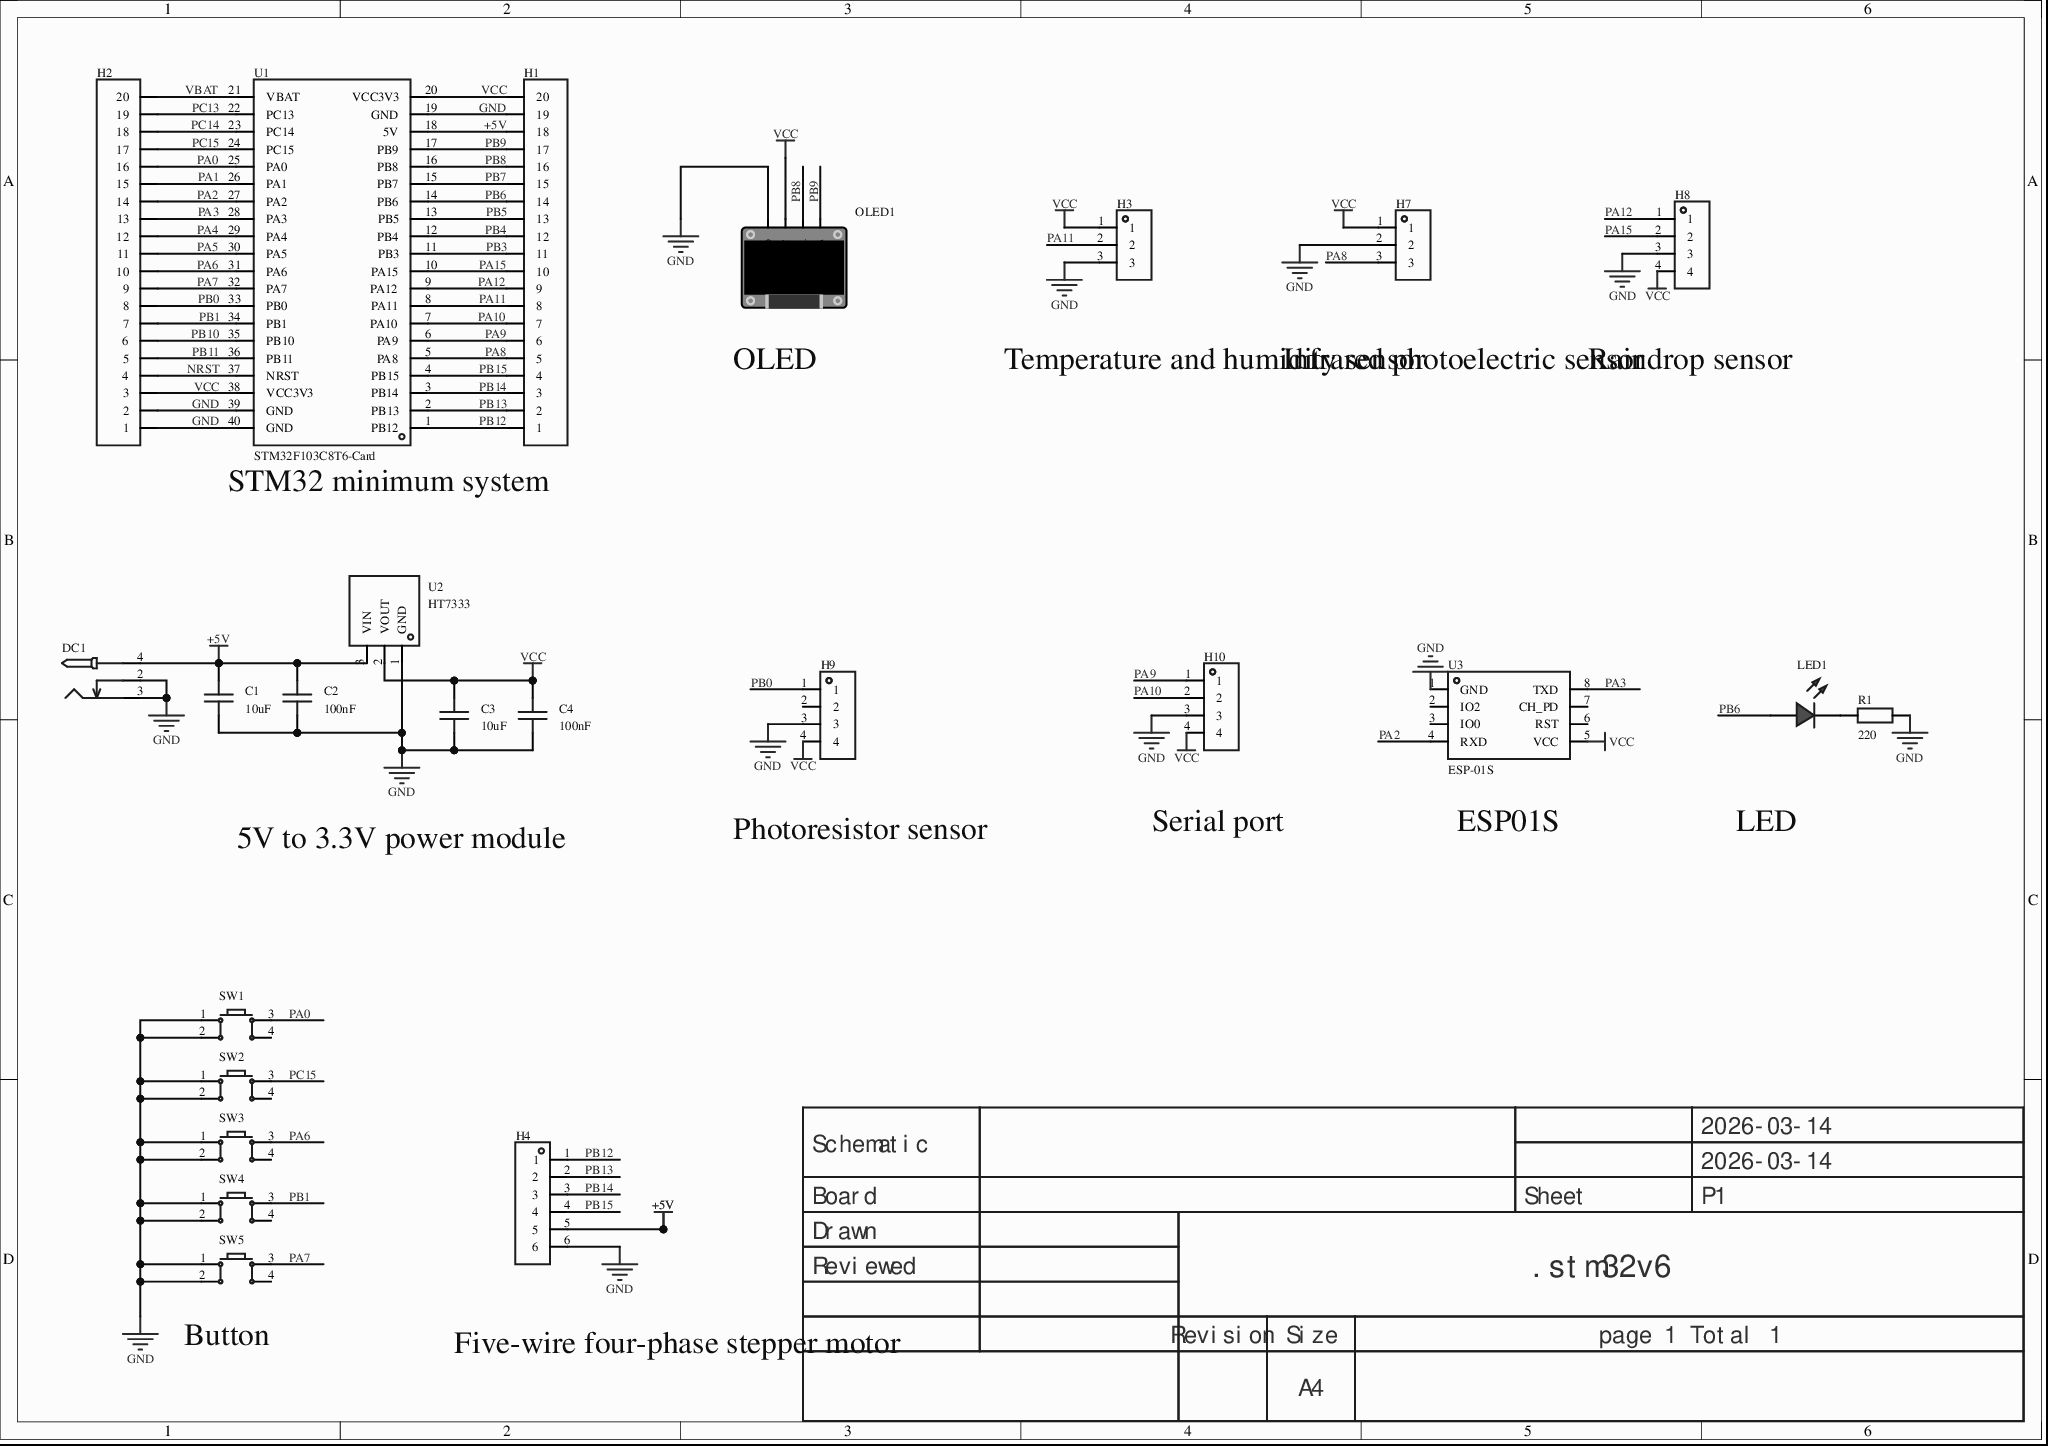
[diagram p0: MISC50760-3.schdoc]
# Altium project MISC50760-2.PrjPcb
1 sheet, 24 parts. Net scope: global (net labels, ports and power ports of the same name join across sheets).
Board file: MISC50760.pcbdoc

## Sheet MISC50760-3.schdoc
size 297 x 209 mm; Version: V1.0; @Project Name: MISC50760; @Page Count: 1; @Update Date: 2026-03-14; @Create Date: 2026-03-14; @Schematic Name: MISC50760; @Page No: 1; @Create Time: 23:22:16; @Update Time: 17:32:40; @Board Name: MISC50760

### Parts
C1  10uF  [C0603]
C2  100nF  [C0603]
C3  10uF  [C0603]
C4  100nF  [C0603]
DC1  (no value)  [DC-2.0]
H1  (no value)  [HDR-TH_20P-P2.54-V-F]
H2  (no value)  [HDR-TH_20P-P2.54-V-F]
H3  (no value)  [HDR-TH_3P-P2.54-V-F]
H4  (no value)  [HDR-TH_6P-P2.54-V-F]
H7  (no value)  [HDR-TH_3P-P2.54-V-F]
H8  (no value)  [HDR-TH_4P-P2.54-V-F]
H9  (no value)  [HDR-TH_4P-P2.54-V-F]
H10  (no value)  [HDR-TH_4P-P2.54-V-F]
LED1  (no value)  [LED_TH-3mm]
OLED1  (no value)  [0.96OLED_4P]
R1  220  [Res_1/8W]
SW1  (no value)  [SW-TH_4P-L6.0-W6.0-P4.50-LS6.5]
SW2  (no value)  [SW-TH_4P-L6.0-W6.0-P4.50-LS6.5]
SW3  (no value)  [SW-TH_4P-L6.0-W6.0-P4.50-LS6.5]
SW4  (no value)  [SW-TH_4P-L6.0-W6.0-P4.50-LS6.5]
SW5  (no value)  [SW-TH_4P-L6.0-W6.0-P4.50-LS6.5]
U1  STM32F103C8T6-Card  [CONN-TH_L53.3-W22.9_STM32F103C8T6-CARD]
U2  HT7333  [SOT-23-3_L2.9-W1.6-P1.90-LS2.8-BR]
U3  ESP-01S  [WIFIM-TH_ESP-01S]

### Nets
+5V: C1.2 C2.2 DC1.4 H1.18 H4.5 U1.18(5V) U2.3(VIN)
GND: C1.1 C2.1 C3.1 C4.1 DC1.2 DC1.3 H1.19 H2.1 H2.2 H3.3 H4.6 H7.2 H8.3 H9.3 H10.3 OLED1.1(GND) R1.2 SW1.1 SW1.2 SW2.1 SW2.2 SW3.1 SW3.2 SW4.1 SW4.2 SW5.1 SW5.2 U1.19(GND) U1.39(GND) U1.40(GND) U2.1(GND) U3.1(GND)
VCC: C3.2 C4.2 H1.20 H2.3 H3.1 H7.1 H8.4 H9.4 H10.4 OLED1.2(VCC) U1.20(VCC3V3) U1.38(VCC3V3) U2.2(VOUT) U3.5(VCC)
NRST: H2.4 U1.37(NRST)
PA0: H2.16 SW1.3 U1.25(PA0)
PA1: H2.15 U1.26(PA1)
PA2: H2.14 U1.27(PA2) U3.4(RXD)
PA3: H2.13 U1.28(PA3) U3.8(TXD)
PA4: H2.12 U1.29(PA4)
PA5: H2.11 U1.30(PA5)
PA6: H2.10 SW3.3 U1.31(PA6)
PA7: H2.9 SW5.3 U1.32(PA7)
PA8: H1.5 H7.3 U1.5(PA8)
PA9: H1.6 H10.1 U1.6(PA9)
PA10: H1.7 H10.2 U1.7(PA10)
PA11: H1.8 H3.2 U1.8(PA11)
PA12: H1.9 H8.1 U1.9(PA12)
PA15: H1.10 H8.2 U1.10(PA15)
PB0: H2.8 H9.1 U1.33(PB0)
PB1: H2.7 SW4.3 U1.34(PB1)
PB3: H1.11 U1.11(PB3)
PB4: H1.12 U1.12(PB4)
PB5: H1.13 U1.13(PB5)
PB6: H1.14 LED1.1(C) U1.14(PB6)
PB7: H1.15 U1.15(PB7)
PB8: H1.16 OLED1.3(SCL) U1.16(PB8)
PB9: H1.17 OLED1.4(SDA) U1.17(PB9)
PB10: H2.6 U1.35(PB10)
PB11: H2.5 U1.36(PB11)
PB12: H1.1 H4.1 U1.1(PB12)
PB13: H1.2 H4.2 U1.2(PB13)
PB14: H1.3 H4.3 U1.3(PB14)
PB15: H1.4 H4.4 U1.4(PB15)
PC13: H2.19 U1.22(PC13)
PC14: H2.18 U1.23(PC14)
PC15: H2.17 SW2.3 U1.24(PC15)
VBAT: H2.20 U1.21(VBAT)
NetLED1_2: LED1.2(A) R1.1

Not connected (* = marked no-connect by the designer): H9 2; SW1 4; SW2 4; SW3 4; SW4 4; SW5 4; U3 2(IO2) 3(IO0) 6(RST) 7(CH_PD)

### Notes on the sheet
- OLED
- Temperature and humidity sensor
- Infrared photoelectric sensor
- Raindrop sensor
- STM32 minimum system
- 5V to 3.3V power module
- Photoresistor sensor
- Serial port
- (near U3) ESP01S
- LED
- (near SW5) Button
- Five-wire four-phase stepper motor
- 2026-03-14
- Schematic
- Board
- Sheet
- P1
- Drawn
- Reviewed
- .stm32v6
- Revision
- Size
- A4
- page 1 Total 1

### Library data of the parts
C1-C4 = CAP_0603: Symbol: Capacitance; ConvertToPcb: yes; ModelId: ac125912035d415993ca9572d50418b10819f05c4eef4c71ace90d822a990e87; ModelName: C0603_L1.6-W0.8-H0.8; ModelTransform: 62.992,31.496,0,0,0,0,0,0,0; Device: CAP_0603; AddInBom: yes; Supplier Footprint: 0603; FootprintName: C0603
  C1 C3: Value: 10uF
  C2 C4: Value: 100nF
DC1 = DC-005_2.0: Symbol: DC power jack; ConvertToPcb: yes; ModelId: f5f20b8a2308479b936ba3c2698865bb0819f05c4eef4c71ace90d822a990e87; ModelName: DC-IN-TH_DC-5520-1; ModelTransform: 372.05,551.18,582.68,90,0,0,137.8,0,-149.61; Device: DC-005_2.0; AddInBom: yes; Supplier Footprint: 插件; FootprintName: DC-2.0
H1 H2 = HDR-F_2.54_1x20P: ConvertToPcb: yes; ModelId: db7015f7ad9d48b8a3b1188db02e3429; ModelName: HDR-F-2.54_1x20; ModelTransform: 1999.996,100,0,0,0,0,0,0,-118.11; Device: HDR-F_2.54_1x20P; Symbol: HDR-F_2.54_1x20P; AddInBom: yes; SupplierPart: C50984; Supplier Footprint: 插件; FootprintName: HDR-TH_20P-P2.54-V-F
H3 H7 = HDR-F_2.54_1x3P: Symbol: PM254V-11-03-H85; ConvertToPcb: yes; ModelId: f3b3cc5aae9641bf9e56fc160cef875b; ModelName: HDR2.54-F-LI-1X3P; ModelTransform: 299.9994,100,0,0,0,0,0,0,-118.11; Device: HDR-F_2.54_1x3P; AddInBom: yes; SupplierPart: C541850; Supplier Footprint: 插件; FootprintName: HDR-TH_3P-P2.54-V-F
H4 = HDR-F_2.54_1x6P: Symbol: Header-Female-2.54_1x6; 3D Model: 0f5bcf94dcda47d085f24cdca1696fe9; 3D Model Transform: 619.684,94.488,0,0,0,0,0,0,-125.984; ConvertToPcb: yes; Device: HDR-F_2.54_1x6P; Supplier Part: C40877; Supplier Footprint: 插件; AddInBom: yes; FootprintName: HDR-TH_6P-P2.54-V-F; ModelName: HDR-TH_6P-P2.54-V-F
H8-H10 = HDR-F_2.54_1x4P: Symbol: 2.54-1*4P female; ConvertToPcb: yes; ModelId: d187812051054f85879fcaa51a310d8e0819f05c4eef4c71ace90d822a990e87; ModelTransform: 419.6842,98.464,0,0,0,0,0,0,-118.11; Device: HDR-F_2.54_1x4P; AddInBom: yes; SupplierPart: C2718488; Supplier Footprint: 插件; FootprintName: HDR-TH_4P-P2.54-V-F; ModelName: HDR-TH_4P-P2.54-V-F
LED1 = LED_TH-R_3mm: ConvertToPcb: yes; ModelId: a497c992633541038a38947cdc58012f0819f05c4eef4c71ace90d822a990e87; ModelName: LED-TH-3mm_R; ModelTransform: 141.274,153.327,0,0,0,0,-5.984,0,-137.795; Symbol: LED_TH-R; Device: LED_TH-R_3mm; AddInBom: yes; FootprintName: LED_TH-3mm; Supplier Footprint: 插件
OLED1 = 0.96OLED模块_4P: Symbol: 0.96OLED module_4P; ConvertToPcb: yes; ModelId: 79c000fdb68d45a296c2e9bedf4f9055; ModelTransform: 1393.69792,1318.895,0,0,0,0,0,-560.079,-137.795; Device: 0.96OLED module_4P; AddInBom: yes; FootprintName: 0.96OLED_4P; Supplier Footprint: 插件; ModelName: 0.96OLED_4P
R1 = Res_AXIAL-1/8W: Symbol: Resistor; ConvertToPcb: yes; ModelId: b2b5ae7ae4c642178fe0039925c86a3f0819f05c4eef4c71ace90d822a990e87; ModelName: RES-TH_BD1.8-L3.2-P7.20-D0.4; ModelTransform: 282.86,66.88,253.09,0,0,0,0,0,-191; Device: Res_AXIAL-1/8W; Value: 220; AddInBom: yes; Supplier Footprint: 轴向引线; FootprintName: Res_1/8W
SW1-SW5 = Key_TH_6x6x6: 触点电流:50mA;额定电压(DC):12V;绝缘电阻:100MΩ;电路结构:单刀单掷;安装方式:直插;按钮形状:圆形按钮;按钮/盖帽颜色:黑色;作用力:260gf@±30gf;工作温度:-25℃~+70℃;引脚样式:PC引脚;开关长度:6mm;开关宽度:6mm;开关高度:6mm;带支架:否;; Symbol: Tactile switch; AddInBom: yes; ModelId: 20eee248bc684ccd8cbdbb1d0d91ec6f0819f05c4eef4c71ace90d822a990e87; ModelName: SW-TH_4P-L6.0-W6.0-H5.0-LS6.5-P4.50; ModelTransform: 236.22,323.03,0,90,0,0,0,0,-137.795; Device: Key_TH_6x6x6; ConvertToPcb: yes; FootprintName: SW-TH_4P-L6.0-W6.0-P4.50-LS6.5; Supplier Footprint: 插件
U1 = STM32F103C8T6-Card: AddInBom: yes; Symbol: STM32F103C8T6-CARD; Device: STM32F103C8T6-Card; LCSC Part Name: STM32F103C8T6-Card; SupplierPart: C9900077949; ManufacturerPart: STM32F103C8T6-Card; Supplier Footprint: 插件; Supplier: LCSC; ConvertToPcb: yes; FootprintName: CONN-TH_L53.3-W22.9_STM32F103C8T6-CARD
U2 = HT7333: Output type: fixed; Operating voltage: 12V; Output voltage: 3.3V; Output current: 250mA; Ripple rejection (PSRR): -; Output polarity: positive;; Manufacturer: 国芯佳品; Symbol: HT7333_C2684634; AddInBom: yes; ModelId: 89cb27a44ab2466697082bb9fd73a7d00819f05c4eef4c71ace90d822a990e87; ModelName: SOT-23-3L_L2.9-W1.6-H1.1-LS2.8-P0.95; ModelTransform: 114.173,110.236,0,90,0,0,0,0,0; Voltage Dropout: 90mV@(40mA); standby current: 2uA; Number of Outputs: 1; Device: HT7333; LCSC Part Name: LDO线性稳压器; SupplierPart: C2684634; ManufacturerPart: HT7333; Supplier Footprint: SOT-23-3L; JLCPCB Part Class: Extended Part; Datasheet: https://item.szlcsc.com/datasheet/HT7333/2783241.html; Supplier: LCSC; ConvertToPcb: yes; FootprintName: SOT-23-3_L2.9-W1.6-P1.90-LS2.8-BR; Output Type: Fixed; Voltage - Supply: 12V; Output Voltage: 3.3V; Output Current: 250mA; Power Supply Rejection Ratio (PSRR): -; Operating Temperature: -25℃~+70℃@(Ta); Output Configuration: Positive
U3 = ESP-01S_C111009: AddInBom: yes; ModelId: eb7175da78ae48b3b1568cfe3027405f0819f05c4eef4c71ace90d822a990e87; ModelTransform: 582.676,976.37608,0,0,0,0,0,388.346,-118.11; Symbol: ESP-01S; Device: ESP-01S_C111009; LCSC Part Name: ESP-01S; SupplierPart: C111009; ManufacturerPart: ESP-01S; Supplier Footprint: -; JLCPCB Part Class: Extended Part; Supplier: LCSC; ConvertToPcb: yes; FootprintName: WIFIM-TH_ESP-01S; ModelName: WIFIM-TH_ESP-01S